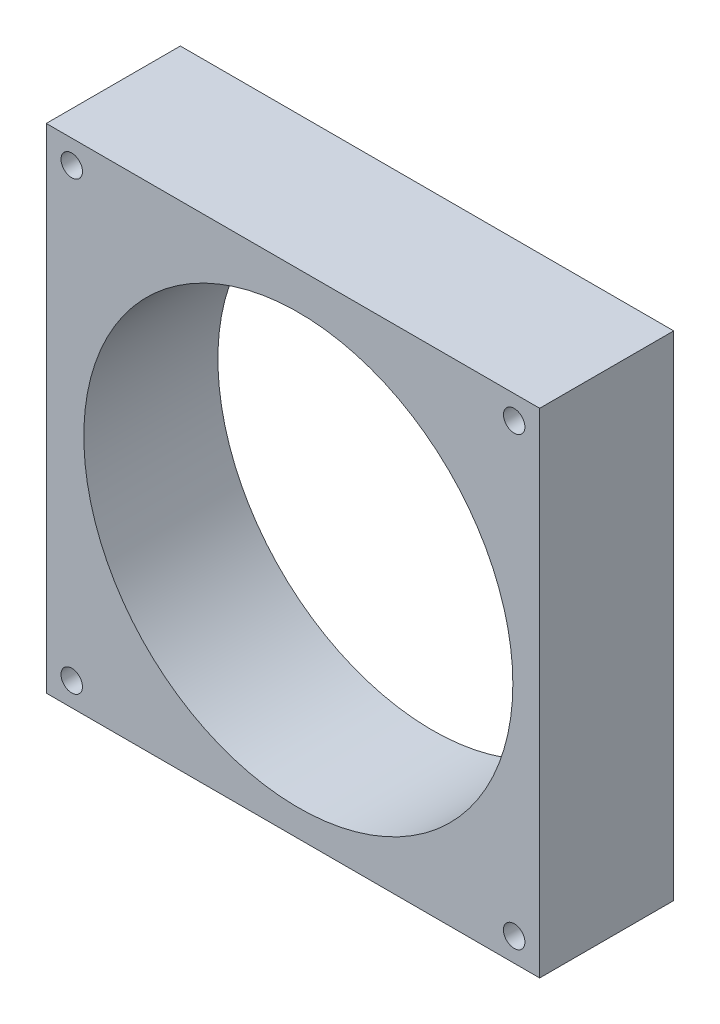
SolidWorks part; units mm, degrees
ref_plane "Front Plane" through (0, 0, 0) normal (0, 0, 1) x (1, 0, 0)
ref_plane "Top Plane" through (0, 0, 0) normal (0, 1, 0) x (1, 0, 0)
ref_plane "Right Plane" through (0, 0, 0) normal (1, 0, 0) x (0, 0, -1)
sketch "Sketch1" plane through (0, 0, 0) normal (0, 0, 1) x (1, 0, 0)
  line L1 (0, 0) -> (-92, 0)
  line L2 (0, 0) -> (0, 92)
  line L3 (0, 92) -> (-92, 92)
  line L4 (-92, 0) -> (-92, 92)
  dimension "D1" = 92
  dimension "D2" = 92
extrude "Boss-Extrude1" add sketch "Sketch1" along normal blind 25
sketch "Sketch2" plane through (0, 0, 25) normal (0, 0, 1) x (1, 0, 0)
  circle A0 centre (-45, 45) radius 40
  dimension "D1" = 80
extrude "Cut-Extrude1" cut sketch "Sketch2" against normal blind 25
sketch "Sketch3" plane through (0, 0, 25) normal (0, 0, 1) x (1, 0, 0)
  line L0 (-46, 92) -> (-46, 0) construction
  line L1 (0, 92) -> (-92, 92) construction
  line L2 (-92, 0) -> (0, 0) construction
  line L3 (-46, 0) -> (-46, 46) construction
  line L4 (-46, 46) -> (0, 46) construction
  line L5 (0, 0) -> (0, 92) construction
  circle A2 centre (-4.75, 87.5998) radius 2
  circle A3 centre (-87.25, 87.5998) radius 2
  circle A4 centre (-87.25, 4.4002) radius 2
  circle A5 centre (-4.75, 4.4002) radius 2
  dimension "D2" = 4
  dimension "D3" = 82.5
  dimension "D1" = 4
extrude "Cut-Extrude2" cut sketch "Sketch3" against normal blind 30
